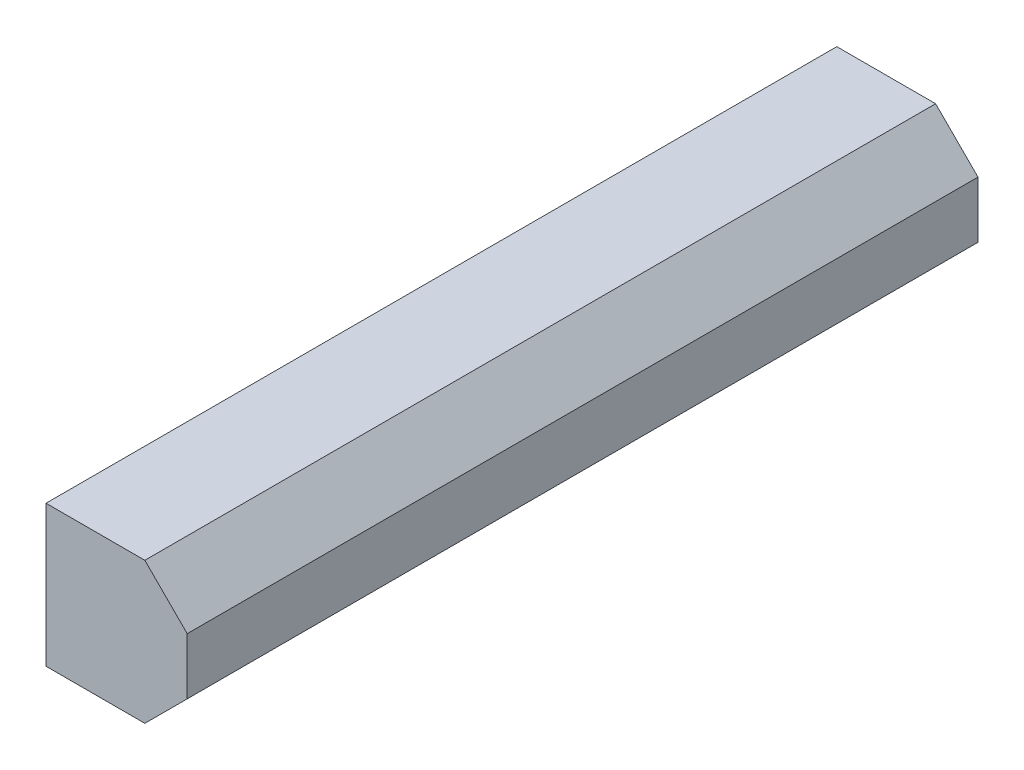
SolidWorks part; units mm, degrees
material "Q235-A"
ref_plane "Front Plane" through (0, 0, 0) normal (0, 0, 1) x (1, 0, 0)
ref_plane "Top Plane" through (0, 0, 0) normal (0, 1, 0) x (1, 0, 0)
ref_plane "Right Plane" through (0, 0, 0) normal (1, 0, 0) x (0, 0, -1)
sketch "Sketch1" plane through (0, 0, 0) normal (1, 0, 0) x (0, 0, -1)
  line L1 (140, -25) -> (-140, -25)
  line L2 (140, -25) -> (140, 25)
  line L3 (140, 25) -> (-140, 25)
  line L4 (-140, -25) -> (-140, 25)
  line L5 (140, -25) -> (-140, 25) construction
  line L6 (140, 25) -> (-140, -25) construction
  point P0 (0, 0)
  dimension "D1" = 50
  dimension "D2" = 280
extrude "Boss-Extrude1" add sketch "Sketch1" along normal mid plane 50
chamfer "Chamfer1" distance 15 angle 45 2 edges at (25, -25, 0) (25, 25, 0)
